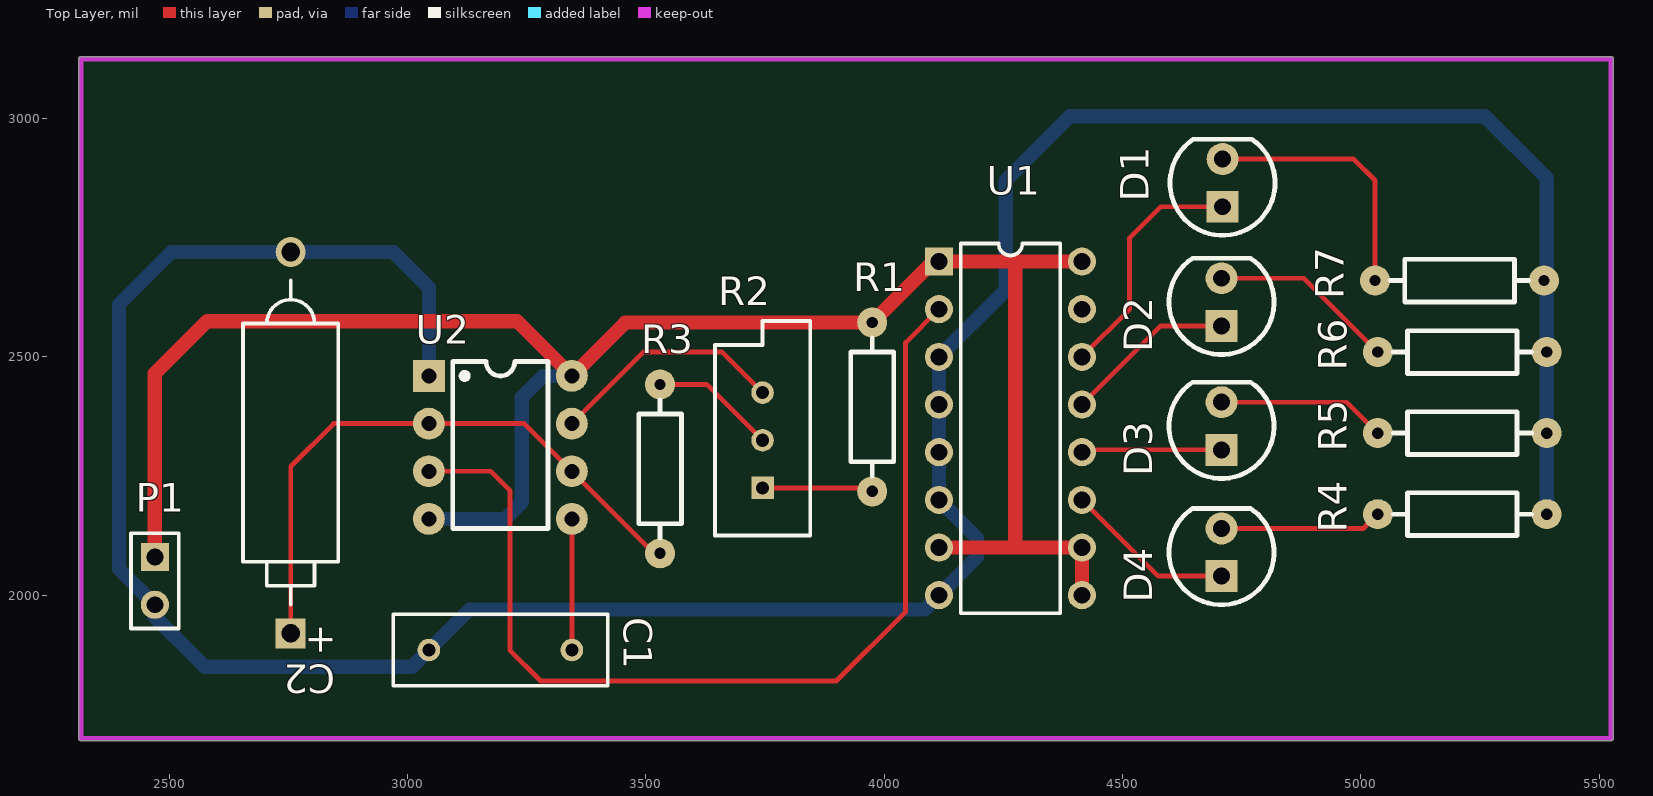
[diagram p0: Top Layer view]
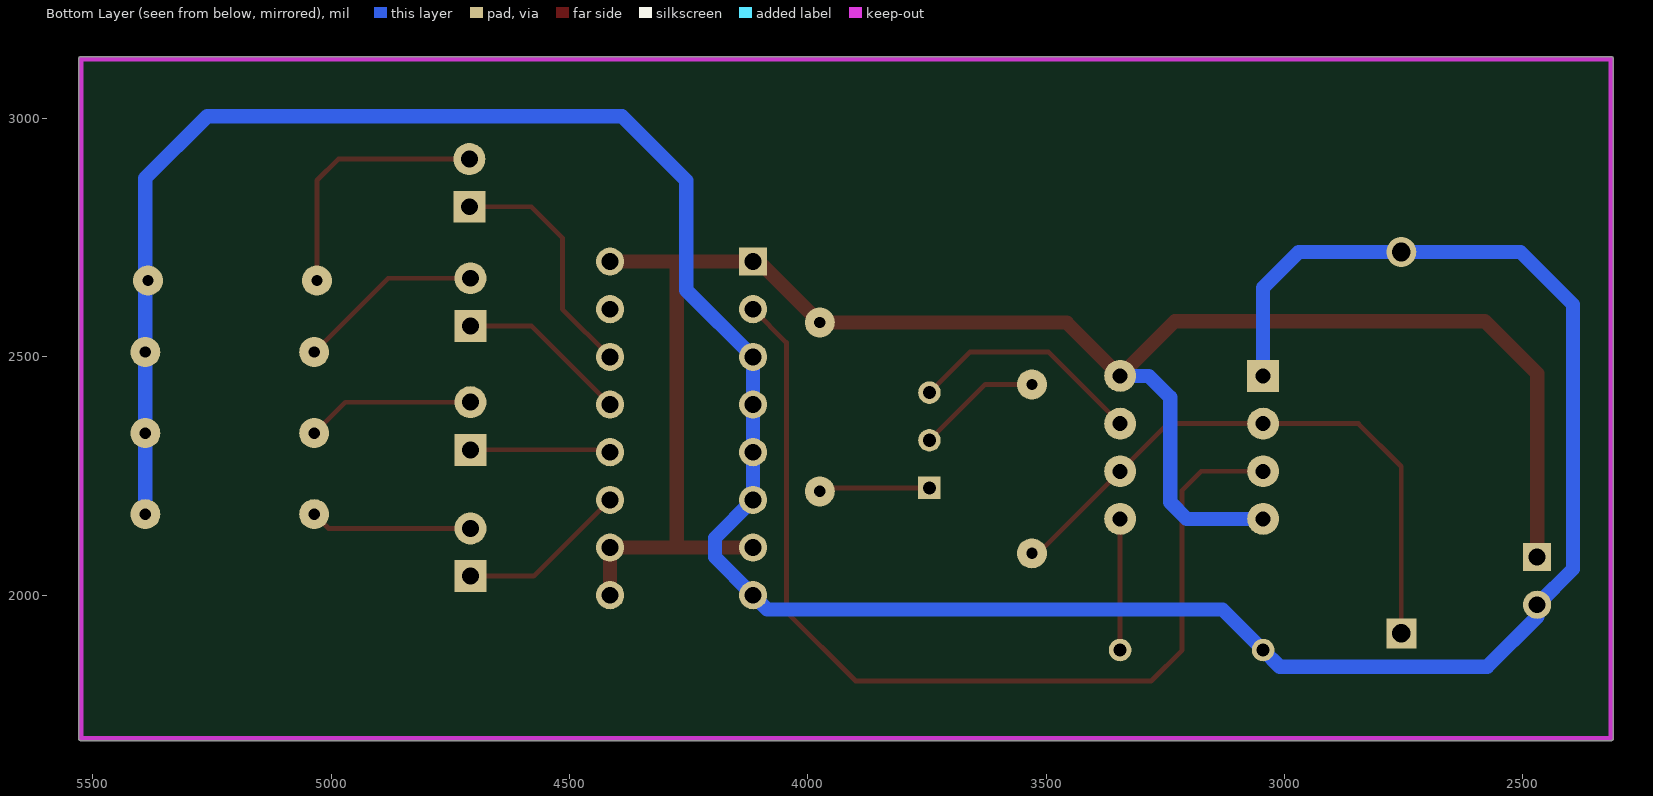
[diagram p1: Bottom Layer view, seen from below]
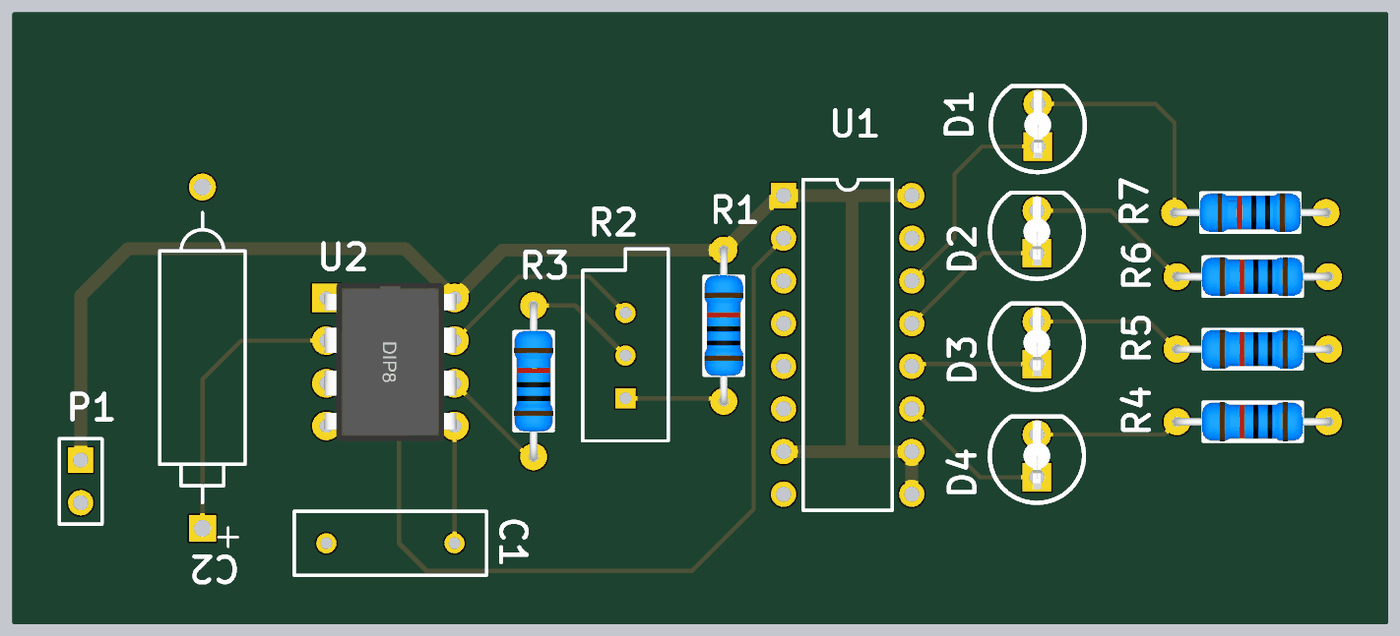
[diagram p2: 3D render of the assembled board from above, using the file's embedded part models]
# Altium PCB MISC82778.PcbDoc
Units mil, origin at the board's own origin, x right, y up, seen from the top; angles counter-clockwise.
Board outline 3220.03 x 1435.03 mil, 2 copper layers (Top Layer, Bottom Layer); 16 components, 16 nets, 53 pads, 0 vias.

## Layer stack, top to bottom (the 12.6 mil dielectric is the usual default, probably not edited)
Top Solder: solder mask 0.4, Solder Resist, Dk 3.5
Top Layer: signal copper 1.4
Dielectric 1: dielectric 12.6, FR-4, Dk 4.8
Bottom Layer: signal copper 1.4
Bottom Solder: solder mask 0.4, Solder Resist, Dk 3.5

## Board outline
2309.99,1700 ccw(c2315,1700) 2315,1694.98 5525,1694.98 ccw(c5525,1700) 5530.02,1700 5530.02,3125 ccw(c5525,3125) 5525,3130.01 2315,3130.01 ccw(c2315,3125) 2309.99,3125

## Design rules (kind name [scope] priority, off if disabled: settings)
Clearance [All] p1: gap=10
MinimumSolderMaskSliver [All] p1: minsoldermaskwidth=0
PolygonConnect [All] p1: connectstyle=Relief reliefconductorwidth=10 reliefentries=4 polygonreliefangle="90 Angle" airgapwidth=10
RoutingVias [All] p1: holewidth=28 width=50 viastyle="Through Hole" minholewidth=28 minwidth=50 maxholewidth=28 maxwidth=50
SilkToSilkClearance [All] p1: silktosilkclearance=0
SilkToSolderMaskClearance [IsPad] p1: minsilkscreentomaskgap=0 clearancetoexposedcopper=TRUE
SolderMaskExpansion [All] p1: expansion=4
Width [All] p1: maxlimit=30 minlimit=10 preferedwidth=10
27 further rules are at their usual default settings.

## Components (designator, comment, footprint, x,y, rotation, side; value= is the part's Value field where it differs from the comment)
C1 "0.01U" RAD-0.3 3195,1885 r0 top
C2 "33U" POLAR0.8 2755,2320 r270 top
D1 "LED" "LED 5MM-W" 4710,2865 r90 top
D2 "LED" "LED 5MM-W" 4707.83,2615 r90 top
D3 "LED" "LED 5MM-W" 4707.83,2355 r90 top
D4 "LED" "LED 5MM-W" 4707.83,2090 r90 top
P1 "Header 2" HDR1X2 2470,2080 r270 top
R1 "10K" "RS 1/4W" 3975,2395 r90 top
R2 "20K" VR5 3745,2325 r90 top
R3 "10K" "RS 1/4W" 3530,2265 r90 top
R4 "470" "RS 1/4W" 5212.83,2170 r180 top
R5 "470" "RS 1/4W" 5212.83,2340 r180 top
R6 "470" "RS 1/4W" 5212.83,2510 r180 top
R7 "470" "RS 1/4W" 5207.17,2660 r180 top
U1 "SN74LS160AN" 648-08 4265,2350 r270 top
U2 "NE555D" DIP8 3195,2310 r0 top

## Footprints (in the part's own frame and the unit in brackets; to place one, negate y for a bottom-side part, rotate by r counter-clockwise, add the part's x,y. Pads: shape width x height; smd on the part's side, far side on the other; paste and mask are expansions set on the pad)
648-08 [mm] "DIP; 16 Leads; Row Spacing 7.62 mm; Pitch 2.54 mm"
  rect 1.5x1.5 hole 0.9: 1(-8.89,-3.81)
  round 1.5 hole 0.9: 2(-6.35,-3.81) 3(-3.81,-3.81) 4(-1.27,-3.81) 5(1.27,-3.81) 6(3.81,-3.81) 7(6.35,-3.81) 8(8.89,-3.81) 9(8.89,3.81) 10(6.35,3.81) 11(3.81,3.81) 12(1.27,3.81) 13(-1.27,3.81) 14(-3.81,3.81) 15(-6.35,3.81) 16(-8.89,3.81)
  silkscreen extent -9.85,-2.65 9.85,2.65
DIP8 [mm]
  rect 1.7x1.7 hole 0.8: 1(-3.81,3.81)
  round 1.7 hole 0.8: 2(-3.81,1.27) 3(-3.81,-1.27) 4(-3.81,-3.81) 5(3.81,-3.81) 6(3.81,-1.27) 7(3.81,1.27) 8(3.81,3.81)
  silkscreen extent -2.54,-4.32 2.54,4.57, body extent -3.94,-4.7 3.91,4.7, height 4.5
HDR1X2 [mm] "Connector; Header; 2 Position"
  rect 1.5x1.5 hole 0.9: 1(0,0)
  round 1.5 hole 0.9: 2(2.54,0)
  silkscreen extent -1.27,-1.27 3.81,1.27
"LED 5MM-W" [mm] "白色5mm直插LED"
  rect 1.7x1.7 hole 0.9: 1(-1.27,0)
  round 1.7 hole 0.9: 2(1.27,0)
  silkscreen extent -2.8,-2.8 2.33,2.8, body extent -2.85,-2.85 2.45,2.85, height 8.75
POLAR0.8 [mm] "Polarized Capacitor; 2 Leads"
  rect 1.6x1.6 hole 1: 1(10.16,0)
  round 1.6 hole 1: 2(-10.16,0)
  silkscreen extent -8.64,-2.54 8.64,2.54
RAD-0.3 [mm] "Radial Cap, Thru-Hole; 2 Leads; 0.3 in Pin Spacing"
  round 1.2 hole 0.7: 1(-3.81,0) 2(3.81,0)
  silkscreen extent -5.71,-1.91 5.71,1.91
"RS 1/4W" [mm] "直插色环电阻，脚距9mm，直径2.3mm"
  round 1.6 hole 0.6: 1(-4.5,0) 2(4.5,0)
  silkscreen extent -3.68,-1.14 3.68,1.14, body extent -4.72,-1.16 4.73,1.16, height 2.32
VR5 [mm] "Thru-Hole; 3 Leads"
  rect 1.2x1.2 hole 0.7: 1(-2.54,0)
  round 1.2 hole 0.7: 2(0,0) 3(2.54,0)
  silkscreen extent -5.08,-2.54 6.35,2.54

## Part data
C1: library part Cap, "Capacitor"
C2: library part "Cap Pol2", "Polarized Capacitor (Axial)"
D1 D2 D3 D4: "Light-emitting diode"
P1: "Header, 2-Pin"
R1 R3 R4 R5 R6 R7: library part R-S, "Color-band resistor"
R2: library part RPot, "Potentiometer"
U1: "BCD Decade Counter"
U2: "General-Purpose Single Bipolar Timer"

## Nets (pads, with @x,y where several pads share a name; then routed paths per layer and width w, separated by ;. In a path a pad name is that pad's centre, name@x,y a point inside that pad or via, vN(x,y) a via of type N, cw(c..) or ccw(c..) an arc to the next point about the centre after c; other vN are vias at no path point)
CLK: U1.2 U2.3 | length 2102.5
  Top Layer w10: U2.3 3175,2260 3215,2220 3215,1885 3280,1820 3900,1820 4045,1965 4045,2530 U1.2
DISC: R2.3 U2.7 | length 497.3
  Top Layer w10: U2.7 3495,2510 3660,2510 R2.3
GND: C1.1 C2.2 P1.2 R4.1 R5.1 R6.1 R7.1 U1.3 U1.4 U1.5 U1.6 U1.8 U2.1 | length 6292.4
  Bottom Layer w30: U2.1 3045,2645 2970,2720 C2.2 2505,2720 2395,2610 2395,2055 P1.2 2470,1955 2575,1850 3010,1850 C1.1 3130,1970 4085,1970 U1.8 4195,2080 4195,2120 U1.6 U1.5 U1.4 U1.3 4255,2640 4255,2870 4390,3005 5260,3005 5390,2875 R6.1 R5.1 R4.1
NetC1_2: C1.2 U2.5 | length 275
  Top Layer w10: C1.2 U2.5
NetC2_1: C2.1 R3.1 U2.2 U2.6 | length 1275
  Top Layer w10: C2.1 2755,2270 2845,2360 U2.2 3245,2360 U2.6 3517.17,2087.83 R3.1
NetD1_1: D1.1 U1.14 | length 513.3
  Top Layer w10: U1.14 4515,2600 4515,2750 4580,2815 D1.1
NetD1_2: D1.2 R7.2 | length 548.6
  Top Layer w10: D1.2 4985,2915 5030,2870 R7.2
NetD2_1: D2.1 U1.13 | length 361.2
  Top Layer w10: U1.13 4580,2565 D2.1
NetD2_2: D2.2 R6.2 | length 392
  Top Layer w10: D2.2 4880.67,2665 R6.2
NetD3_1: D3.1 U1.12 | length 294.9
  Top Layer w10: U1.12 4420,2305 D3.1
NetD3_2: D3.2 R5.2 | length 354.8
  Top Layer w10: D3.2 4970.67,2405 R5.2
NetD4_1: D4.1 U1.11 | length 359.1
  Top Layer w10: U1.11 4575,2040 D4.1
NetD4_2: D4.2 R4.2 | length 340.3
  Top Layer w10: D4.2 5005.67,2140 R4.2
NetR1_1: R1.1 R2.1 | length 233
  Top Layer w10: R2.1 3967.83,2225 R1.1
NetR2_2: R2.2 R3.2 | length 263.5
  Top Layer w10: R3.2 3627.83,2442.17 R2.2
VCC: P1.1 R1.2 U1.1 U1.7 U1.9 U1.10 U1.16 U2.4 U2.8 | length 4075.7
  Top Layer w30: P1.1 2470,2465 2580,2575 3230,2575 U2.8 3457.17,2572.17 R1.2 4102.83,2700 U1.1 4275,2700 ; U1.7 4275,2100 ; U1.9 U1.10 4275,2100 ; U1.16 4275,2700 ; 4275,2100 4275,2700
  Bottom Layer w30: U2.4 3205,2160 3240,2195 3240,2415 3285,2460 U2.8
pads on no net: U1.15

## Keep-outs
Keep-Out Layer:
  lines w10: 2315,1700 2315,3105 2315,3125 5525,3125 5525,3100 5525,1700 2315,1700